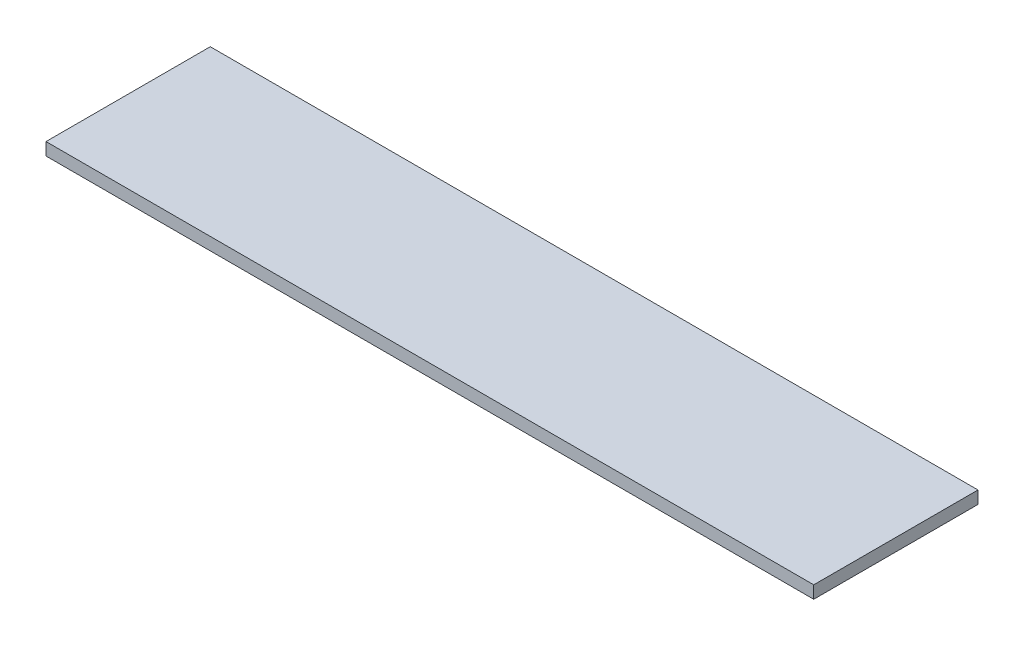
from build123d import *

# Parameters (mm, degrees)
SKETCH_1_W      = 1346
SKETCH_1_H      = 288
EXTRUDE_1_DEPTH = 20
SHELL_1_T       = -2
SKETCH_2_W      = 1346
SKETCH_2_H      = 288
EXTRUDE_2_DEPTH = 2


with BuildPart() as part:
    # 草图1 → 凸台-拉伸1 (new body)
    with BuildSketch(Plane(origin=(0, 0, 0), x_dir=(1, 0, 0), z_dir=(0, 1, 0))):
        Rectangle(SKETCH_1_W, SKETCH_1_H)
    extrude(amount=-EXTRUDE_1_DEPTH)

    # 抽壳1
    shell_1_openings = [part.faces().sort_by_distance(p)[0] for p in [
        (0, -20, 0),
    ]]
    offset(amount=SHELL_1_T, openings=shell_1_openings, kind=Kind.INTERSECTION)

    # 草图2 → 凸台-拉伸2 (add)
    with BuildSketch(Plane.XZ.offset(20)):
        Rectangle(SKETCH_2_W, SKETCH_2_H)
    extrude(amount=EXTRUDE_2_DEPTH)


solid = part.part
